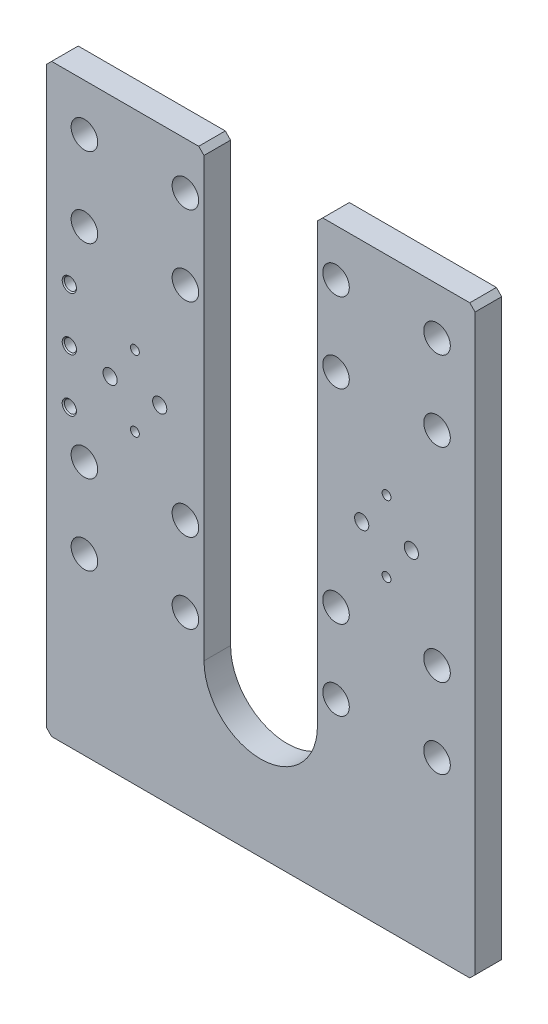
SolidWorks part; units mm, degrees
material "Q235-A"
ref_plane "Front Plane" through (0, 0, 0) normal (0, 0, 1) x (1, 0, 0)
ref_plane "Top Plane" through (0, 0, 0) normal (0, 1, 0) x (1, 0, 0)
ref_plane "Right Plane" through (0, 0, 0) normal (1, 0, 0) x (0, 0, -1)
sketch "Sketch1" plane through (0, 0, 0) normal (0, 0, 1) x (1, 0, 0)
  line L0 (3.0212, 249.1385) -> (3.0212, -207.8999) construction
  line L1 (-117.9788, 156.5901) -> (-28.9788, 156.5901)
  line L2 (-117.9788, 156.5901) -> (-117.9788, -173.4099)
  line L3 (-117.9788, -173.4099) -> (124.0212, -173.4099)
  line L4 (124.0212, 156.5901) -> (124.0212, -173.4099)
  line L6 (-28.9788, 156.5901) -> (-28.9788, -93.4099)
  line L8 (35.0212, 156.5901) -> (35.0212, -93.4099)
  line L9 (35.0212, 156.5901) -> (124.0212, 156.5901)
  arc A0 (-28.9788, -93.4099) -> (35.0212, -93.4099) centre (3.0212, -93.4099) ccw
  dimension "D1" = 242
  dimension "D2" = 330
  dimension "D4" = 64
  dimension "D5" = 32
extrude "Boss-Extrude1" add sketch "Sketch1" along normal blind 15
chamfer "Chamfer1" distance 3 angle 45 6 edges at (-117.9788, -173.4099, 7.5) (124.0212, -173.4099, 7.5) (124.0212, 156.5901, 7.5) (35.0212, 156.5901, 7.5) (-28.9788, 156.5901, 7.5) (-117.9788, 156.5901, 7.5)
sketch "Sketch2" plane through (0, 0, 15) normal (0, 0, 1) x (1, 0, 0)
  line L0 (3.0212, -191.2803) -> (3.0212, 199.1743) construction
  line L1 (-104.9788, 52.5901) -> (-104.9788, -7.4099)
  line L2 (-96.4788, 130.0522) -> (-39.4788, 130.0522)
  line L3 (-96.4788, 130.0522) -> (-96.4788, 85.0522)
  line L4 (-96.4788, 85.0522) -> (-39.4788, 85.0522)
  line L5 (-39.4788, 130.0522) -> (-39.4788, 85.0522)
  line L6 (-81.9788, 19.0901) -> (-53.9788, 19.0901)
  line L7 (-114.9788, -173.4099) -> (121.0212, -173.4099) construction
  line L9 (-96.4788, -29.9478) -> (-39.4788, -29.9478)
  line L10 (-39.4788, -29.9478) -> (-39.4788, -74.9478)
  line L11 (-96.4788, -29.9478) -> (-96.4788, -74.9478)
  line L12 (-96.4788, -74.9478) -> (-39.4788, -74.9478)
  line L13 (102.5212, -74.9478) -> (45.5212, -74.9478)
  line L14 (102.5212, -29.9478) -> (102.5212, -74.9478)
  line L15 (45.5212, -29.9478) -> (45.5212, -74.9478)
  line L16 (102.5212, -29.9478) -> (45.5212, -29.9478)
  line L17 (88.0212, 19.0901) -> (60.0212, 19.0901)
  line L18 (45.5212, 130.0522) -> (45.5212, 85.0522)
  line L19 (102.5212, 85.0522) -> (45.5212, 85.0522)
  line L20 (102.5212, 130.0522) -> (102.5212, 85.0522)
  line L21 (102.5212, 130.0522) -> (45.5212, 130.0522)
  line L23 (-117.9788, 153.5901) -> (-117.9788, -170.4099) construction
  circle A0 centre (-104.9788, 22.5901) radius 6.7182
  point P18 (-67.9788, -74.9478)
  dimension "D1" = 45
  dimension "D2" = 57
  dimension "D3" = 99.5
  dimension "D4" = 60
  dimension "D5" = 28
  dimension "D6" = 192.5
  dimension "D7" = 85
  dimension "D8" = 205
  dimension "D9" = 166
  dimension "D10" = 13
hole_wizard "Hole1" positions "Sketch3" profile "Sketch4" legacy end condition through all
sketch "Sketch3" plane through (0, 0, 15) normal (0, 0, 1) x (1, 0, 0)
  point P0 (-96.4788, 130.0522)
  point P3 (-39.4788, 130.0522)
  point P6 (-39.4788, 85.0522)
  point P9 (-96.4788, 85.0522)
  point P12 (-96.4788, -29.9478)
  point P15 (-39.4788, -29.9478)
  point P18 (-39.4788, -74.9478)
  point P21 (-96.4788, -74.9478)
  point P24 (45.5212, -74.9478)
  point P27 (45.5212, -29.9478)
  point P30 (102.5212, -29.9478)
  point P33 (102.5212, -74.9478)
  point P36 (45.5212, 85.0522)
  point P39 (45.5212, 130.0522)
  point P42 (102.5212, 130.0522)
  point P45 (102.5212, 85.0522)
sketch "Sketch4" plane through (-96.4788, 130.0522, 15) normal (1, 0, 0) x (0, -1, 0)
  line L0 (0, 0) -> (0, 15)
  line L1 (0, 15) -> (4.5, 15)
  line L2 (4.5, 15) -> (4.5, 10.6)
  line L3 (4.5, 10.6) -> (7.5, 10.6)
  line L4 (7.5, 10.6) -> (7.5, 0)
  line L5 (7.5, 0) -> (0, 0)
  line L6 (0, 110) -> (0, -10) construction
  dimension "直径" = 9
  dimension "深度" = 15
  dimension "柱坑直径" = 15
  dimension "柱坑深度" = 10.6
hole_wizard "M8 Tapped Hole1" positions "Sketch5" profile "Sketch6" tap size "M8" standard "GB" end condition through all
sketch "Sketch5" plane through (0, 0, 15) normal (0, 0, 1) x (1, 0, 0)
  point P0 (-104.9788, 52.5901)
  point P3 (-104.9788, 22.5901)
  point P6 (-104.9788, -7.4099)
sketch "Sketch6" plane through (-104.9788, 52.5901, 15) normal (1, 0, 0) x (0, -1, 0)
  line L0 (0, 0) -> (0, 15)
  line L1 (0, 15) -> (3.4, 15)
  line L2 (3.4, 15) -> (3.4, 0.625)
  line L3 (3.4, 0.625) -> (4.025, 0)
  line L5 (4.025, 0) -> (0, 0)
  line L6 (-3.4, 0.625) -> (-4.025, 0) construction
  line L11 (0, -6.35) -> (0, 107.95) construction
  dimension "通孔螺纹孔钻头直径" = 6.8
  dimension "通孔螺纹孔钻头深度" = 15
  dimension "近端锥形沉头孔直径" = 8.05
  dimension "近端锥形沉头孔角度" = 90
cosmetic thread "Cosmetic thread 4" parameters "D2"=8
cosmetic thread "Cosmetic thread 5" parameters "D2"=8
cosmetic thread "Cosmetic thread 6" parameters "D2"=8
hole_wizard "Hole2" positions "Sketch7" profile "Sketch8" legacy
sketch "Sketch7" plane through (0, 0, 15) normal (0, 0, 1) x (1, 0, 0)
  point P0 (-81.9788, 19.0901)
  point P3 (-53.9788, 19.0901)
  point P6 (60.0212, 19.0901)
  point P9 (88.0212, 19.0901)
sketch "Sketch8" plane through (-81.9788, 19.0901, 15) normal (1, 0, 0) x (0, -1, 0)
  line L0 (0, 0) -> (0, 8)
  line L1 (0, 8) -> (4, 8)
  line L2 (4, 8) -> (4, 0)
  line L3 (4, 0) -> (0, 0)
  line L4 (0, 110) -> (0, -10) construction
  dimension "直径" = 8
  dimension "深度" = 8
sketch "Sketch9" plane through (0, 0, 0) normal (0, 0, -1) x (-1, 0, 0)
  line L0 (-3.0212, -190.3694) -> (-3.0212, 158.5192) construction
  line L1 (114.9788, -173.4099) -> (-121.0212, -173.4099) construction
  line L2 (-74.0212, 39.0901) -> (67.9788, 39.0901)
  line L3 (-74.0212, 39.0901) -> (-74.0212, -0.9099)
  line L4 (-74.0212, -0.9099) -> (67.9788, -0.9099)
  line L5 (67.9788, 39.0901) -> (67.9788, -0.9099)
  dimension "D1" = 142
  dimension "D2" = 40
  dimension "D3" = 71
  dimension "D4" = 172.5
hole_wizard "M6 Tapped Hole1" positions "Sketch10" profile "Sketch11" tap size "M6" standard "GB" end condition through all
sketch "Sketch10" plane through (0, 0, 0) normal (0, 0, -1) x (-1, 0, 0)
  point P0 (-74.0212, 39.0901)
  point P3 (-74.0212, -0.9099)
  point P6 (67.9788, -0.9099)
  point P9 (67.9788, 39.0901)
sketch "Sketch11" plane through (74.0212, 39.0901, 0) normal (1, 0, 0) x (0, 1, 0)
  line L0 (0, 0) -> (0, 15)
  line L1 (0, 15) -> (2.5, 15)
  line L2 (2.5, 15) -> (2.5, 0)
  line L5 (2.5, 0) -> (0, 0)
  line L11 (0, -6.35) -> (0, 107.95) construction
  dimension "通孔螺纹孔钻头直径" = 5
  dimension "通孔螺纹孔钻头深度" = 15
cosmetic thread "Cosmetic thread 7" parameters "D2"=6
cosmetic thread "Cosmetic thread 8" parameters "D2"=6
cosmetic thread "Cosmetic thread 9" parameters "D2"=6
cosmetic thread "Cosmetic thread 10" parameters "D2"=6
